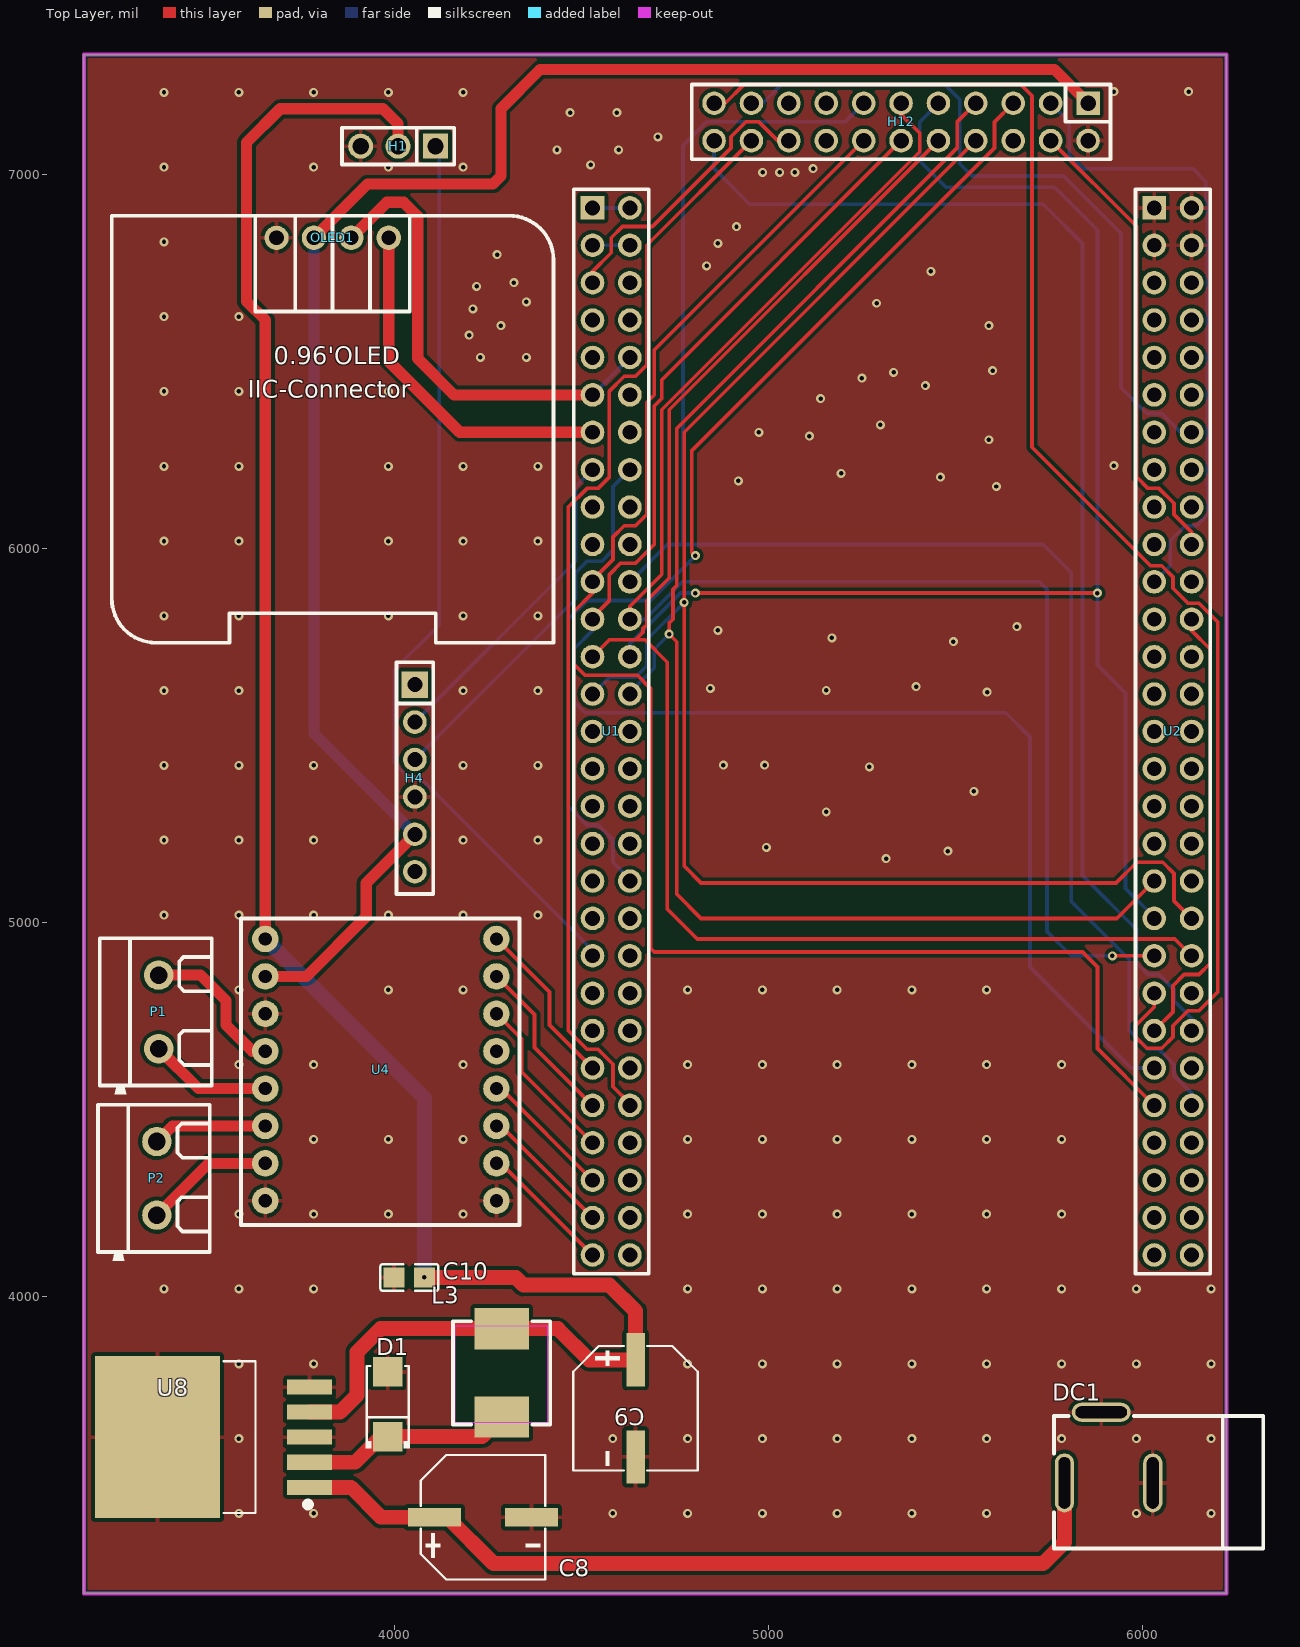
[diagram p0: Top Layer view]
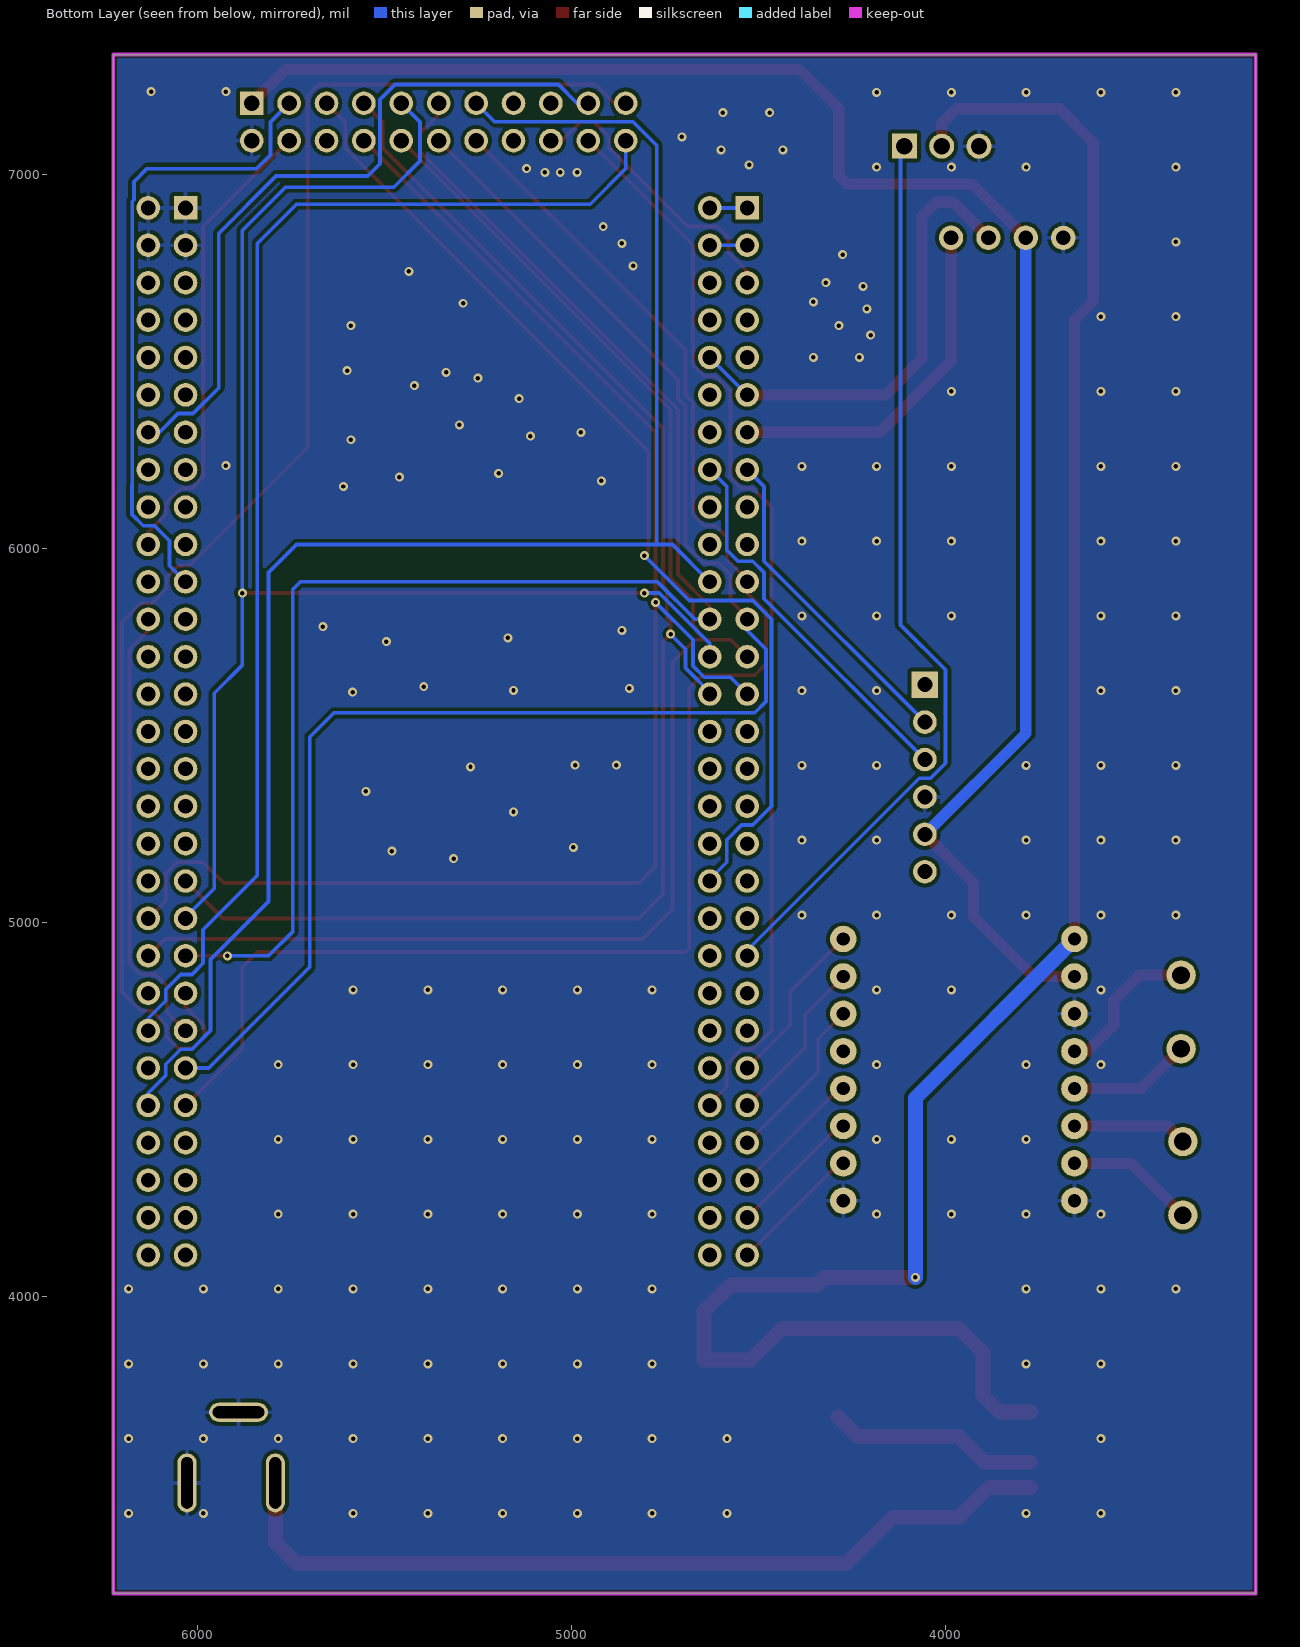
[diagram p1: Bottom Layer view, seen from below]
# Altium PCB MISC51443.pcbdoc
Units mil, origin at the board's own origin, x right, y up, seen from the top; angles counter-clockwise.
Board outline 3055 x 4115 mil, 2 copper layers (Top Layer, Bottom Layer), stack 62.206 mil thick; 16 components, 110 nets, 190 pads, 191 vias.

## Layer stack, top to bottom
Top Solder Mask Layer: solder mask 0.394, Dk 3.3
Top Layer: signal copper 1.379
Dielectric1: surface 59.449, FR4, Dk 4.5
Bottom Layer: signal copper 1.378
Bottom Solder Mask Layer: solder mask 0.394, Dk 3.3

## Board outline
3170,7320 3170,3205 6225,3205 6225,7320

## Design rules (kind name [scope] priority, off if disabled: settings)
BoardOutlineClearance copperThickness2oz_1 [All] p2 off: genericclearance=7.99 ignorepadtopadclearanceinfootprint=FALSE except(0: Arc-SplitContinuation Track-SplitContinuation SMDPad-SplitContinuation THPad-SplitContinuation Via-SplitContinuation Fill-SplitContinuation Region-SplitContinuation Poly-SplitContinuation Text-SplitContinuation Hole-SplitContinuation; 5.98: Arc-CutoutEdge SMDPad-CutoutEdge THPad-CutoutEdge Via-CutoutEdge Fill-CutoutEdge Region-CutoutEdge Text-CutoutEdge; 6.93: Hole-OutlineEdge Hole-CutoutEdge; 10: Poly-OutlineEdge Poly-CutoutEdge; 11.81: Arc-OutlineEdge Track-OutlineEdge SMDPad-OutlineEdge THPad-OutlineEdge Via-OutlineEdge Fill-OutlineEdge Region-OutlineEdge Text-OutlineEdge Track-CutoutEdge)
BoardOutlineClearance copperThickness1oz_1 [All] p4: genericclearance=4.02 ignorepadtopadclearanceinfootprint=FALSE except(0: Arc-SplitContinuation Track-SplitContinuation SMDPad-SplitContinuation THPad-SplitContinuation Via-SplitContinuation Fill-SplitContinuation Region-SplitContinuation Poly-SplitContinuation Text-SplitContinuation Hole-SplitContinuation; 6: SMDPad-CutoutEdge THPad-CutoutEdge Via-CutoutEdge Fill-CutoutEdge Region-CutoutEdge Text-CutoutEdge; 6.93: Hole-OutlineEdge Hole-CutoutEdge; 10: Poly-OutlineEdge Poly-CutoutEdge; 11.8: Arc-OutlineEdge Track-OutlineEdge SMDPad-OutlineEdge THPad-OutlineEdge Via-OutlineEdge Fill-OutlineEdge Region-OutlineEdge Text-OutlineEdge; 11.81: Arc-CutoutEdge Track-CutoutEdge)
Clearance copperThickness2oz [All] p1 off: gap=7.99 ignorepadtopadclearanceinfootprint=FALSE except(5.98: SMDPad-Track SMDPad-SMDPad THPad-Track SMDPad-THPad THPad-THPad Track-Via SMDPad-Via THPad-Via Via-Via Fill-Track Region-Track Fill-SMDPad Region-SMDPad Fill-THPad Region-THPad Fill-Via Region-Via Fill-Fill Fill-Region Region-Region Arc-Track Arc-SMDPad Arc-THPad Arc-Via Fill-Arc Region-Arc Arc-Arc Text-Track SMDPad-Text Text-THPad Text-Via Fill-Text Region-Text Arc-Text Text-Text; 6.93: Hole-Track Hole-SMDPad Hole-THPad Hole-Via Fill-Hole Region-Hole Hole-Arc Hole-Text; 10: Poly-Track Poly-SMDPad Poly-THPad Poly-Via Poly-Fill Poly-Region Poly-Poly Poly-Arc Poly-Text Poly-Hole)
Clearance copperThickness1oz [All] p3: gap=4.02 ignorepadtopadclearanceinfootprint=FALSE except(5.98: SMDPad-Track SMDPad-SMDPad THPad-Track SMDPad-THPad THPad-THPad Track-Via SMDPad-Via THPad-Via Via-Via Fill-Track Region-Track Fill-SMDPad Region-SMDPad Fill-THPad Region-THPad Fill-Via Region-Via Fill-Fill Fill-Region Region-Region; 6: Arc-Track Arc-SMDPad Arc-THPad Arc-Via Fill-Arc Region-Arc Arc-Arc Text-Track SMDPad-Text Text-THPad Text-Via Fill-Text Region-Text Arc-Text Text-Text; 6.93: Hole-Track Hole-SMDPad Hole-THPad Hole-Via Fill-Hole Region-Hole Hole-Arc Hole-Text; 10: Poly-Track Poly-SMDPad Poly-THPad Poly-Via Poly-Fill Poly-Region Poly-Poly Poly-Arc Poly-Text Poly-Hole)
DiffPairsRouting differentialPair [All] p1: maxlimit=6 minlimit=6 mostfreqgap=6 toplayer_minwidth=5 toplayer_prefwidth=10 toplayer_maxwidth=100 toplayer_mingap=6 toplayer_prefgap=6 toplayer_maxgap=6 bottomlayer_minwidth=5 bottomlayer_prefwidth=10 bottomlayer_maxwidth=100 bottomlayer_mingap=6 bottomlayer_prefgap=6 bottomlayer_maxgap=6 maxuncoupledlength=10
HoleToHoleClearance otherClearance [All] p1: gap=11.81 allowstackedmicrovias=TRUE
Length netLength [All] p1: minlimit=0 maxlimit=0
MatchedLengths netLengthTolerance [All] p1: tolerance=1000
PasteMaskExpansion pasteMaskExpansion [All] p1: expansion=0
PlaneConnect innerPlane [All] p1: planeconnectstyle=Relief reliefexpansion=20 reliefentries=4 reliefconductorwidth=10 reliefairgap=10
PolygonConnect copperRegion [(InNet('GND'))] p1: connectstyle=Relief reliefconductorwidth=10 reliefentries=4 polygonreliefangle="90 Angle" airgapwidth=10 via.connectstyle=Relief via.reliefconductorwidth=10 via.reliefentries=4 via.polygonreliefangle="90 Angle" via.airgapwidth=10
RoutingVias viaSize [All] p1: holewidth=12.01 width=24.02 viastyle="Through Hole" minholewidth=11.81 minwidth=19.68 maxholewidth=248.03 maxwidth=393.7
SolderMaskExpansion solderMaskExpansion [IsVia] p1: expansion=-1000 istentingtop=TRUE
SolderMaskExpansion solderMaskExpansion [All] p2: expansion=2 istentingtop=FALSE
Width copperThickness2oz_2 [All] p1 off: maxlimit=100 minlimit=8 preferedwidth=10
Width copperThickness1oz_2 [All] p2: maxlimit=100 minlimit=5 preferedwidth=10

## Components (designator, comment, footprint, x,y, rotation, side; value= is the part's Value field where it differs from the comment)
C8 "" CAP-SMD_BD8.0-L8.3-W8.3-RD 4237.11,3408.75 r180 top
C9 "" CAP-SMD_BD8.0-L8.3-W8.3-RD 4645,3700 r90 top
C10 "" C0805 4040,4050 r180 top
D1 "" SMA_L4.3-W2.6-LS5.2-RD 3982.11,3710.75 r90 top
DC1 "" DC-2.0 5915,3490 r0 top
H1 "" HDR-TH_3P-P2.54-V-M 4010,7075 r180 top
H4 "" HDR-TH_6P-P2.54-V-F 4055,5385 r270 top
H12 "DS1023-2*11SF11" HDR-TH_22P-P2.54-V-F-R2-C11-S2.54 5355,7140 r180 top
L3 "" IND-SMD_L7.0-W6.6 4287.11,3794.75 r90 top
OLED1 "" 0.96OLED_4P 3835,6830 r0 top
P1 "KF301-2P接线端子" CONN-TH_XY301V-A-5.0-2P 3370,4760 r270 top
P2 "KF301-2P接线端子" CONN-TH_XY301V-A-5.0-2P 3365,4315 r270 top
U1 "KH-2.54FH-2X29P-H8.5" HDR-TH_58P-P2.54-V-F-R2-C29-S2.54 4580,5510 r270 top
U2 "KH-2.54FH-2X29P-H8.5" HDR-TH_58P-P2.54-V-F-R2-C29-S2.54 6081.97,5510 r270 top
U4 "" tb6612 3655,4955 r0 top
U8 "LM2596S-5.0" TO-263-5_L10.2-W8.9-P1.70-BR 3569.98,3622.75 r0 top

## Footprints (in the part's own frame and the unit in brackets; to place one, negate y for a bottom-side part, rotate by r counter-clockwise, add the part's x,y. Pads: shape width x height; smd on the part's side, far side on the other; paste and mask are expansions set on the pad)
0.96OLED_4P [mm]
  round 1.65 hole 1 copper offset 0,0: 1(-3.81,-0.001) 2(-1.27,0.002) 3(1.27,0.002) 4(3.81,0.002)
  silkscreen extent -15,-27.5 15,1.5
C0805 [mm]
  rect 1.41x1.35 smd paste-100 mask+0.051: 1(-1.03,0) 2(1.03,0)
  silkscreen extent -1.96,-0.9 1.96,0.9
CAP-SMD_BD8.0-L8.3-W8.3-RD [mm]
  rect 3.61x1.26 smd paste+0 mask+0.051: 1(3.295,0) 2(-3.295,0)
  silkscreen extent -4.23,-4.23 4.23,4.23
CONN-TH_XY301V-A-5.0-2P [mm]
  round 2 hole 1.2: 1(-2.5,0) 2(2.5,0)
  silkscreen extent -5,-4 5.6,3.6
DC-2.0 [mil]
  oval 157.5x51.2 hole 31.5 slot 137.8 at 0 deg paste+0 mask+2: 2(-24.7,199.5)
  oval 51.2x157.5 hole 31.5 slot 137.8 at 90 deg paste+0 mask+2: 3(113.1,10.5) 4(-123.1,10.5)
  silkscreen extent -151,-165 408,190
HDR-TH_3P-P2.54-V-M [mm]
  rect 1.7x1.7 hole 1.1: 1(-2.54,0)
  round 1.7 hole 1.1: 2(0,0) 3(2.54,0)
  silkscreen extent -3.81,-1.25 3.81,1.25
HDR-TH_6P-P2.54-V-F [mm]
  rect 1.8x1.8 hole 1.02: 1(-6.35,0)
  round 1.6 hole 1.02: 2(-3.81,0) 3(-1.27,0) 4(1.27,0) 5(3.81,0) 6(6.35,0)
  silkscreen extent -7.87,-1.25 7.87,1.25
HDR-TH_22P-P2.54-V-F-R2-C11-S2.54 [mm]
  rect 1.6x1.6 hole 1.05: 1(-12.7,-1.27)
  round 1.6 hole 1.05: 2(-12.7,1.27) 3(-10.16,-1.27) 4(-10.16,1.27) 5(-7.62,-1.27) 6(-7.62,1.27) 7(-5.08,-1.27) 8(-5.08,1.27) 9(-2.54,-1.27) 10(-2.54,1.27) 11(0,-1.27) 12(0,1.27) 13(2.54,-1.27) 14(2.54,1.27) 15(5.08,-1.27) 16(5.08,1.27) 17(7.62,-1.27) 18(7.62,1.27) 19(10.16,-1.27) 20(10.16,1.27) 21(12.7,-1.27) 22(12.7,1.27)
  silkscreen extent -14.22,-2.54 14.22,2.54
HDR-TH_58P-P2.54-V-F-R2-C29-S2.54 [mm]
  rect 1.6x1.6 hole 1: 1(-35.56,-1.27)
  round 1.6 hole 1: 2(-35.56,1.27) 3(-33.02,-1.27) 4(-33.02,1.27) 5(-30.48,-1.27) 6(-30.48,1.27) 7(-27.94,-1.27) 8(-27.94,1.27) 9(-25.4,-1.27) 10(-25.4,1.27) 11(-22.86,-1.27) 12(-22.86,1.27) 13(-20.32,-1.27) 14(-20.32,1.27) 15(-17.78,-1.27) 16(-17.78,1.27) 17(-15.24,-1.27) 18(-15.24,1.27) 19(-12.7,-1.27) 20(-12.7,1.27) 21(-10.16,-1.27) 22(-10.16,1.27) 23(-7.62,-1.27) 24(-7.62,1.27) 25(-5.08,-1.27) 26(-5.08,1.27) 27(-2.54,-1.27) 28(-2.54,1.27) 29(0,-1.27) 30(0,1.27) 31(2.54,-1.27) 32(2.54,1.27) 33(5.08,-1.27) 34(5.08,1.27) 35(7.62,-1.27) 36(7.62,1.27) 37(10.16,-1.27) 38(10.16,1.27) 39(12.7,-1.27) 40(12.7,1.27) 41(15.24,-1.27) 42(15.24,1.27) 43(17.78,-1.27) 44(17.78,1.27) 45(20.32,-1.27) 46(20.32,1.27) 47(22.86,-1.27) 48(22.86,1.27) 49(25.4,-1.27) 50(25.4,1.27) 51(27.94,-1.27) 52(27.94,1.27) 53(30.48,-1.27) 54(30.48,1.27) 55(33.02,-1.27) 56(33.02,1.27) 57(35.56,-1.27) 58(35.56,1.27)
  silkscreen extent -36.83,-2.54 36.83,2.54
IND-SMD_L7.0-W6.6 [mil]
  rect 110.2x145.7 smd paste+0 mask+2: 1(-118.1,0) 2(118.1,0)
  silkscreen extent -138,-130 138,130
SMA_L4.3-W2.6-LS5.2-RD [mm]
  rect 2x2 smd paste+0 mask+0.051: 1(-2.2,0) 2(2.2,0)
  silkscreen extent -2.98,-1.5 2.6,1.5
tb6612 [mm]
  round 1.8 hole 0.9: 1(0,0) 2(0,-2.54) 3(0,-5.08) 4(0,-7.62) 5(0,-10.16) 6(0,-12.7) 7(0,-15.24) 8(0,-17.78) 9(15.697,-17.78) 10(15.697,-15.24) 11(15.697,-12.7) 12(15.697,-10.16) 13(15.697,-7.62) 14(15.697,-5.08) 15(15.697,-2.54) 16(15.697,0)
TO-263-5_L10.2-W8.9-P1.70-BR [mm]
  rect 3.083x1.02 smd: 1(5.16,-3.4) 2(5.16,-1.7) 3(5.16,0) 4(5.16,1.7) 5(5.16,3.4)
  rect 8.5x11 smd: 6(-5.16,0)
  silkscreen extent -0.66,-5.16 5.26,5.16

## Via types
v1: diameter 24.02, hole 12, Top Layer to Bottom Layer, 191 vias

## Nets (pads, with @x,y where several pads share a name; then routed paths per layer and width w, separated by ;. In a path a pad name is that pad's centre, name@x,y a point inside that pad or via, vN(x,y) a via of type N, cw(c..) or ccw(c..) an arc to the next point about the centre after c; other vN are vias at no path point)
3V3: U1.3 U1.4 | length 100
  Bottom Layer w10: U1.3 U1.4
5V: U1.1 U1.2 | length 100
  Bottom Layer w10: U1.1 U1.2
$1N219: P1.1 U4.4 | length 407.3
  Top Layer w30: P1.1 3481.57,4858.43 3550,4790 3550,4725 3620,4655 U4.4
$1N220: P1.2 U4.5 | length 329.1
  Top Layer w30: P1.2 3476.57,4555 U4.5
$1N221: P2.1 U4.6 | length 307.2
  Top Layer w30: P2.1 3406.57,4455 U4.6
$1N222: P2.2 U4.7 | length 347.3
  Top Layer w30: P2.2 3503.43,4355 U4.7
$1N241: C8.1 DC1.4 U8.1 | length 2285.4
  Top Layer w40: U8.1 3884.45,3488.89 3964.59,3408.75 C8.1 4141.25,3408.75 4265,3285 5735,3285 5791.9,3341.9 DC1.4
$1N246: D1.1 L3.1 U8.2 | length 545.4
  Top Layer w40: U8.2 3895.19,3555.82 D1.1@3963.51,3624.14 ; D1.1 4234.6,3624.14 L3.1
+5V: C9.1 C10.1 H1.2 L3.2 U4.1 U8.4 | length 5549
  Top Layer w30: U4.1 3655,6610 3605,6660 3605,7085 3695,7175 3970,7175 4010,7135 H1.2
  Top Layer w40: U8.4 3854.68,3689.68 3900,3735 3900,3850 3962.85,3912.85 L3.2 4437.15,3912.85 4520.28,3829.72 C9.1 4645,3960 4575,4030 4345,4030 4325,4050 v1(4080.55,4050)
  Bottom Layer w40: U4.1 4080.55,4529.45 v1(4080.55,4050)
A0: H12.14 U1.21 U2.49 | length 4314.2
  Top Layer w10: H12.14 4695,6530 4695,6410 4675,6390 4675,6090 4645,6060 4615,6060 4585,6030 4585,5970 4530,5915 U1.21 4530,5880 4480,5830 4480,5690 4510,5660 4650,5660 4685,5625 4685,4930 4695,4920 5840,4920 5880,4880 5880,4661.97 U2.49
A1: H12.13 U1.22 U2.50 | length 4425.2
  Bottom Layer w10: U1.22 4730,6010 4772.12,6010 ; H12.13 5205,7140 4835,7140 4772.12,7077.12 4772.12,6010 ; U2.50 6131.97,4543.04 6085,4590 6085,4620 6045,4660 6015,4660 5965,4710 5965,4900 5810,5055 5810,5935 5735,6010 4772.12,6010
A2: H12.12 U1.23 U2.47 | length 4204
  Top Layer w10: U1.23 4530,5815 4575,5860 4575,5930 4605,5960 4645,5960 4695,6010 4695,6380 4715,6400 4715,6450 H12.12
  Bottom Layer w10: U1.23 4530,5780 4480,5730 4480,5590 4510,5560 5635,5560 5700,5495 5700,4880 5970,4610 U2.47
A3: H12.11 U1.24 U2.41 | length 4115.3
  Top Layer w10: U1.24 4630,5845 4715,5930 4715,6370 5405,7060 5405,7110 5355,7160 H12.11 ; v1(5920,4910) U2.41
  Bottom Layer w10: U1.24 4670,5810 4770,5910 5725,5910 5745,5890 5745,4975 5810,4910 v1(5920,4910)
A4: H12.10 U1.25 U2.42 | length 4027.8
  Top Layer w10: U1.25 4575,5755 4645,5755 ; H12.10 4735,6370 4735,5920 4675,5860 4675,5795 4665,5785 4665,5775 4645,5755 ; U2.42 6086.97,4955 4810,4955 4730,5035 4730,5695 4670,5755 4645,5755
A5: H12.9 U1.26 U2.39 | length 3971.2
  Top Layer w10: v1(4805,5880) v1(5880,5880)
  Bottom Layer w10: U1.26 4630,5745 4765,5880 v1(4805,5880) ; H12.9 5405,7140 5405,7035 5475,6965 5765,6965 5880,6850 v1(5880,5880) 5880,5687.35 5955,5612.35 5955,5090 6031.97,5013.04 U2.39
A6: H12.8 U1.27 U2.40 | length 4153.9
  Top Layer w10: H12.8 4775,6310 v1(4775,5855) 4775,5150 4820,5105 5930,5105 5985,5160 6055,5160 6085,5130 6085,5056.97 U2.40
  Bottom Layer w10: U1.27 4575,5655 4645,5655 4675,5685 4675,5755 v1(4775,5855)
A7: H12.7 U1.28 U2.37 | length 4011.7
  Top Layer w10: H12.7 5505,7140 5505,7070 4755,6320 4755,5900 4745,5890 4745,5810 4735,5800 v1(4735,5770) 4755,5750 4755,5075 4820,5010 5931.97,5010 U2.37
  Bottom Layer w10: U1.28 4630,5615 4695,5680 4695,5730 v1(4735,5770)
A8: U1.17
A9: H4.2 U1.15 | length 871.7
  Bottom Layer w10: H4.2 4485,5965 4485,6165 U1.15
A10: H4.3 U1.16 | length 1036.6
  Bottom Layer w10: H4.3 4485,5865 4485,5935 4515,5965 4555,5965 4585,5995 4585,6165 U1.16
A11: H12.18 U1.5 | length 782.4
  Top Layer w10: U1.5 4530,6740 4580,6790 4580,6830 4610,6860 4690,6860 4900,7070 4900,7100 4940,7140 4975,7140 5025,7090 H12.18
A12: U1.6
A15: H12.20 U1.50 | length 2904
  Top Layer w10: U1.50 4630,4515.01 4585,4560 4585,4620 4545,4660 4515,4660 4465,4710 4465,6110 4515,6160 4545,6160 4575,6190 4575,6420 4615,6460 4645,6460 4675,6490 4675,6810 H12.20
B0: H12.21 U2.43 | length 3970.9
  Top Layer w10: H12.21 4885,7190 4935,7240 5675,7240 5705,7210 5705,6270 6021.97,5953.03 6051.97,5953.03 6081.97,5923.03 6081.97,5893.03 6121.97,5853.03 6151.97,5853.03 6201.97,5803.03 6201.97,4813.04 6151.97,4763.04 6121.97,4763.04 6081.97,4723.04 6081.97,4693.04 6051.97,4663.04 6011.97,4663.04 5981.97,4693.04 5981.97,4723.04 6031.97,4773.04 U2.43
B1: H12.22 U2.46 | length 3386.4
  Bottom Layer w10: H12.22 4855,7015 4950,6920 5735,6920 5840,6815 5840,5125 5985,4980 5985,4890 6015,4860 6045,4860 6085,4820 6085,4790 6131.97,4743.04 U2.46
B2: U2.35
B3: U1.33
B4: U1.34
B5: U1.35
B6: U1.36
B7: U1.37
B8: H12.5 U1.38 | length 2766.7
  Top Layer w10: v1(4805,5980) 4795,5990 4795,6260 5605,7070 5605,7140 H12.5
  Bottom Layer w10: U1.38 4630,5115.01 4585,5160 4585,5220 4545,5260 4515,5260 4465,5310 4465,5810 4515,5860 4685,5860 v1(4805,5980)
B9: U1.39
B10: H12.3 U2.21 | length 1702.6
  Bottom Layer w10: H12.3 5805,7140 5805,7051.69 5841.69,7015 6135,7015 6170,6980 6170,6932.04 6174.45,6927.6 6174.45,6169.94 6175,6169.39 6175,6090 6145,6060 6115,6060 6075,6020 6075,5953.03 U2.21
B11: H12.4 U2.20 | length 1253.7
  Top Layer w10: H12.4 5985,6860 5985,6190 6015,6160 6045,6160 6085,6120 6085,6090 6131.97,6043.03 U2.20
B12: H12.19 U2.14 | length 1925.6
  Bottom Layer w10: H12.19 4985,7190 5035,7240 5471.97,7240 5511.97,7200 5511.97,7028.03 5545,6995 5790,6995 5942.86,6842.14 5942.86,6429.11 6011.96,6360 6051.96,6360 6101.96,6310 U2.14
B13: U2.13
B14: U2.12
B15: U2.11
C0: U2.56
C1: U2.55
C2: U2.58
C3: U2.57
C4: U2.38
C5: U2.44
C6: U1.12
C8: U1.14
C9: OLED1.4 U1.13 | length 953.8
  Top Layer w30: OLED1.4@3985,6830.05 3985,6500 4175,6310 U1.13
C10: U1.18
C11: U1.19
C12: U1.20
C13: U1.51 U4.14 | length 451.5
  Top Layer w10: U4.14 4340,4688 4340,4600 U1.51
D8: U2.10
D9: U2.9
D10: U2.8
D11: U2.7
D12: U2.6
D13: U2.5
D14: U2.15
D15: U2.16
E0: H1.1 U1.41 | length 2456
  Bottom Layer w10: H1.1 4120,7065 4120,5795 4000,5675 4000,5425 4040,5385 4070,5385 4530,4925 U1.41
E1: U1.40
E2: U1.45
E3: U1.46
E4: U1.47 U4.16 | length 451.5
  Top Layer w10: U4.16 4415,4813 4415,4725 U1.47
E5: U1.48
E6: U1.49 U4.15 | length 451.5
  Top Layer w10: U4.15 4375,4753 4375,4665 U1.49
E7: U2.29
E8: U2.30
E9: U2.28
E10: U2.27
E11: U2.26
E12: U2.25
E13: U2.24 U2.45 | length 1206.3
  Top Layer w10: U2.45 6081.97,4760 6081.97,4830 6111.97,4860 6151.97,4860 6181.97,4890 6181.97,5730 6131.97,5780 U2.24
E14: U2.23
E15: U2.22
F0: U1.52
F1: U1.53 U4.12 | length 358.5
  Top Layer w10: U4.12 4285,4555 U1.53
F2: U1.54
F3: U1.55 U4.11 | length 358.5
  Top Layer w10: U4.11 4285,4455 U1.55
F4: U1.56
F5: U1.57 U4.10 | length 358.5
  Top Layer w10: U4.10 4285,4355 U1.57
F6: U1.58
F7: U2.52
F8: U2.51
F9: U2.54
F10: U2.53
F11: U2.36
F12: U2.33
F14: U2.48
F15: U2.34
G0: U2.31
G1: U2.32
G2: U2.17
G3: U2.18
G4: U2.19
G5: U1.8
G6: U1.7
G7: OLED1.3 U1.10 U1.11 | length 1261.7
  Top Layer w30: OLED1.3@3885,6830.05 3979.95,6925 4025,6925 4062.58,6887.42 4062.58,6507.42 4160,6410 U1.11
  Bottom Layer w10: U1.11 U1.10
G8: U1.9
G9: U1.29
G10: U1.30
G11: U1.31
G12: U1.44
G13: U1.43
G14: U1.42
G15: U1.32
GND: C8.2 C9.2 C10.2 D1.2 DC1.2 DC1.3 H1.3 H4.4 H12.2 OLED1.1 U2.1 U2.2 U2.3 U2.4 U4.3 U4.8 U4.9 U8.3 U8.5 U8.6
  other v1: 3584.1,3419.1 3784.1,3419.1 4584.1,3419.1 4784.1,3419.1 4984.1,3419.1 5184.1,3419.1 5384.1,3419.1 5584.1,3419.1 5984.1,3419.1 6184.1,3419.1 3584.1,3619.1 4584.1,3619.1 4784.1,3619.1 4984.1,3619.1 5184.1,3619.1 5384.1,3619.1 5584.1,3619.1 5784.1,3619.1 5984.1,3619.1 6184.1,3619.1 3584.1,3819.1 3784.1,3819.1 4784.1,3819.1 4984.1,3819.1 5184.1,3819.1 5384.1,3819.1 5584.1,3819.1 5784.1,3819.1 5984.1,3819.1 6184.1,3819.1 3384.1,4019.1 3584.1,4019.1 3784.1,4019.1 4784.1,4019.1 4984.1,4019.1 5184.1,4019.1 5384.1,4019.1 5584.1,4019.1 5784.1,4019.1 5984.1,4019.1 6184.1,4019.1 3584.1,4219.1 3784.1,4219.1 3984.1,4219.1 4184.1,4219.1 4784.1,4219.1 4984.1,4219.1 5184.1,4219.1 5384.1,4219.1 5584.1,4219.1 5784.1,4219.1 3784.1,4419.1 3984.1,4419.1 4184.1,4419.1 4784.1,4419.1 4984.1,4419.1 5184.1,4419.1 5384.1,4419.1 5584.1,4419.1 5784.1,4419.1 3584.1,4619.1 3784.1,4619.1 4184.1,4619.1 4784.1,4619.1 4984.1,4619.1 5184.1,4619.1 5384.1,4619.1 5584.1,4619.1 5784.1,4619.1 3584.1,4819.1 3984.1,4819.1 4184.1,4819.1 4784.1,4819.1 4984.1,4819.1 5184.1,4819.1 5384.1,4819.1 5584.1,4819.1 3384.1,5019.1 3584.1,5019.1 3784.1,5019.1 3984.1,5019.1 4184.1,5019.1 4384.1,5019.1 5315,5170 5480,5190 4995,5200 3384.1,5219.1 3584.1,5219.1 3784.1,5219.1 4184.1,5219.1 4384.1,5219.1 5155,5295 5550,5350 5270,5415 3384.1,5419.1 3584.1,5419.1 3784.1,5419.1 4184.1,5419.1 4384.1,5419.1 4880,5420 4990,5420 5585,5615 3384.1,5619.1 3584.1,5619.1 4184.1,5619.1 4384.1,5619.1 5155,5620 4845,5625 5395,5630 5495,5750 5170,5760 4865,5780 5665,5790 3384.1,5819.1 3584.1,5819.1 3984.1,5819.1 4184.1,5819.1 4384.1,5819.1 3384.1,6019.1 3584.1,6019.1 3984.1,6019.1 4184.1,6019.1 4384.1,6019.1 5610,6165 4920,6180 5460,6190 5195,6200 3384.1,6219.1 3584.1,6219.1 3984.1,6219.1 4184.1,6219.1 4384.1,6219.1 5924.1,6221.11 5590,6290 5110,6300 4975,6310 5300,6330 5140,6400 3384.1,6419.1 3584.1,6419.1 3984.1,6419.1 5420,6435 5250,6455 5335,6470 5600,6475 4230,6510 4352.98,6510 4200,6570 4285,6595 5590,6595 3384.1,6619.1 3584.1,6619.1 4210,6640 5290,6655 4352.98,6658.61 4220,6700 4320,6710 5435,6740 4835,6755 4275,6785 4865,6815 3384.1,6819.1 4915,6860 4985,7005 5030,7005 5071.25,7005 5120,7015 3384.1,7019.1 3784.1,7019.1 3984.1,7019.1 4184.1,7019.1 4525,7025 4435,7065 4600,7065 4705,7100 4470,7165 4595,7165 3384.1,7219.1 3584.1,7219.1 3784.1,7219.1 3984.1,7219.1 4184.1,7219.1 5924.1,7221.11 6124.1,7221.11
STBY: U4.13
VCC: H4.5 H12.1 OLED1.2 U4.2 | length 4716.1
  Top Layer w30: U4.2 3765,4855 3925,5015 3925,5105 H4.5 ; OLED1.2@3785,6830.05 3928.74,6973.79 4263.79,6973.79 4285,6995 4285,7175 4390,7280 5765,7280 H12.1
  Bottom Layer w30: OLED1.2@3785,6830.05 3785,5505 H4.5
pads on no net: H4.1 H4.6 H12.6 H12.15 H12.16 H12.17

## Polygon pours and split planes (outlines as drawn)
GND on Bottom Layer (solid, remove dead copper, pour order 2): 3050,7495 3050,3090 6590,3090 6590,7495
GND on Top Layer (solid, remove dead copper, pour order 0): 3000,7515 3000,3000 6535,3000 6535,7515

## Keep-outs
Top Layer:
  region: 4161.51,3918.85 4161.51,3663.35 4410.01,3663.35 4410.01,3918.85
Board Outline Layer:
  the board outline again, w10

## Silkscreen, mask and mechanical layers (free items; w line width, h text height)
Top Silkscreen Layer:
  lines w10: 3590,4190 3590,5010 4335,5010 4335,4190 3590,4190